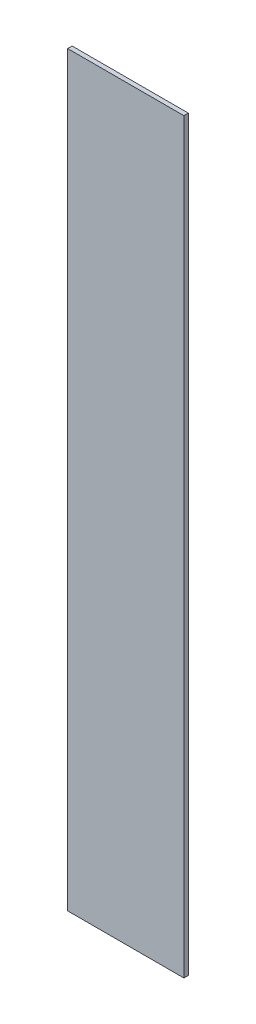
SolidWorks part; units mm, degrees
material "PMMA(有机玻璃)"
ref_plane "前视" through (0, 0, 0) normal (0, 0, 1) x (1, 0, 0)
ref_plane "上视" through (0, 0, 0) normal (0, 1, 0) x (1, 0, 0)
ref_plane "右视" through (0, 0, 0) normal (1, 0, 0) x (0, 0, -1)
sketch "草图1" plane through (0, 0, 0) normal (0, 0, 1) x (1, 0, 0)
  line L1 (-65.5, 421) -> (65.5, 421)
  line L2 (-65.5, 421) -> (-65.5, -421)
  line L3 (-65.5, -421) -> (65.5, -421)
  line L4 (65.5, 421) -> (65.5, -421)
  line L5 (-65.5, 421) -> (65.5, -421) construction
  line L6 (-65.5, -421) -> (65.5, 421) construction
  point P0 (0, 0)
  dimension "D1" = 842
  dimension "D2" = 131
extrude "凸台-拉伸1" add sketch "草图1" along normal blind 5
hole_wizard "M5 间隙孔1" positions "草图3" profile "草图2" hole size "M5" standard "GB"
sketch "草图3" plane through (0, 0, 5) normal (0, 0, 1) x (1, 0, 0)
  line L0 (-427.5, 273) -> (-427.5, -273) construction
  line L1 (-427.5, -273) -> (427.5, -273) construction
  line L2 (0, 273) -> (0, -273) construction
  line L3 (427.5, 273) -> (-427.5, 273) construction
  line L5 (-427.5, 0) -> (427.5, 0) construction
  line L6 (427.5, -273) -> (427.5, 273) construction
  point P0 (-375, -261)
  point P46 (415.5, 250)
  point P48 (-415.5, 250)
  point P58 (-125, -261)
  point P59 (125, -261)
  point P61 (-125, 261)
  point P62 (125, 261)
  point P64 (-375, 261)
  point P88 (375, -261)
  point P89 (375, 261)
  point P108 (415.5, 0)
  point P109 (-415.5, 0)
  point P110 (415.5, -250)
  point P111 (-415.5, -250)
  dimension "D1" = 12
  dimension "D2" = 12
  dimension "D5" = 3
  dimension "D3" = 12
  dimension "D6" = 4
  dimension "D4" = 2
sketch "草图2" plane through (-375, -261, 5) normal (1, 0, 0) x (0, -1, 0)
  line L0 (0, 0) -> (0, 5)
  line L1 (0, 5) -> (2.75, 5)
  line L2 (2.75, 5) -> (2.75, 0)
  line L5 (2.75, 0) -> (0, 0)
  line L11 (0, -6.35) -> (0, 107.95) construction
  dimension "通孔孔直径" = 5.5
  dimension "通孔孔深度" = 5
